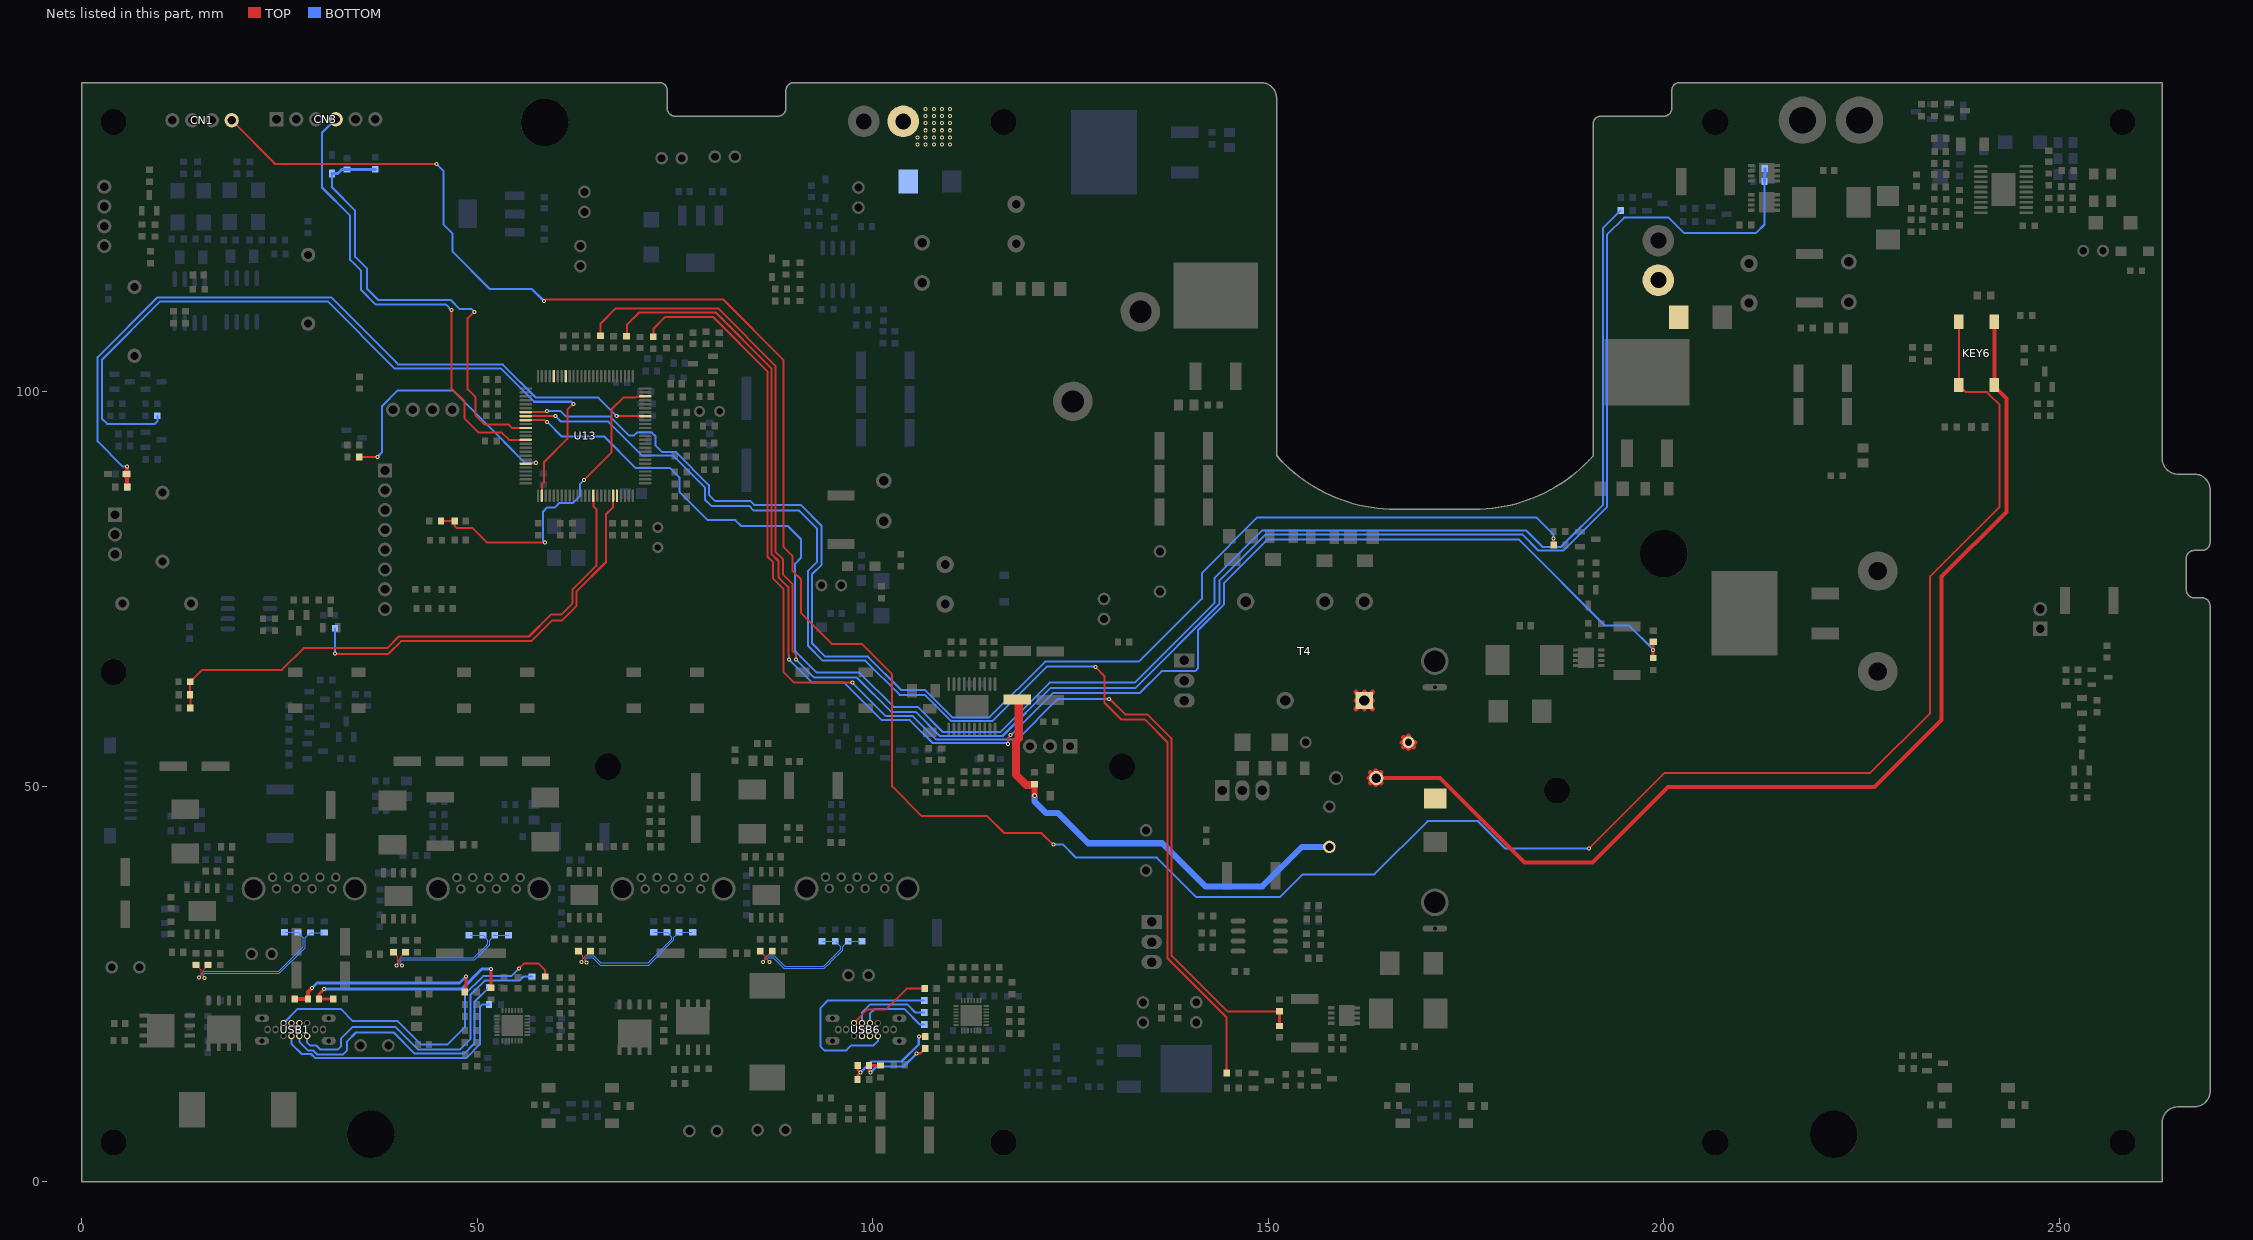
[diagram p0: the nets of this part, all layers, seen from the top]
# Altium PCB MISC84402.PcbDoc (part 4 of 12)
Units mm, origin at the board's own origin, x right, y up, seen from the top; angles counter-clockwise.
Board outline 269.06 x 139 mm, 4 copper layers (TOP, GND02, PWR03, BOTTOM), stack 0.732 mm thick; 694 components, 428 nets, 1859 pads, 1384 vias.

## Via types
v1: diameter 0.508, hole 0.254, TOP to BOTTOM, tented both sides, 1015 vias
v2: diameter 0.508, hole 0.254, TOP to BOTTOM, 243 vias
v3: diameter 0.508, hole 0.305, TOP to BOTTOM, 60 vias
v4: diameter 0.61, hole 0.305, TOP to BOTTOM, 55 vias
v5: diameter 0.61, hole 0.305, TOP to BOTTOM, tented both sides, 8 vias
v6: diameter 0.762, hole 0.381, TOP to BOTTOM, 2 vias
v7: diameter 0.762, hole 0.381, TOP to BOTTOM, tented both sides, 1 vias

## Nets (pads, with @x,y where several pads share a name; then routed paths per layer and width w, separated by ;. In a path a pad name is that pad's centre, name@x,y a point inside that pad or via, vN(x,y) a via of type N, cw(c..) or ccw(c..) an arc to the next point about the centre after c; other vN are vias at no path point) (continued)
BAT1+: C98.2 C125.1 F6.2 KEY6.3 KEY6.4 R13.2 R16.2 R20.1 T4.1 | length 218.9
  TOP w0.508: C98.2@163.906,51.105 171.679,51.105 182.397,40.386 190.983,40.386 200.508,49.911 226.644,49.911 235.128,58.395 235.128,76.556 243.307,84.734 243.307,99.06 241.798,100.569 KEY6.3@241.798,100.75 KEY6.4@241.798,108.75
  TOP w0.635: T4.1@161.074,59.82 T4.1@162.125,60.871 ; T4.1@161.074,60.871 T4.1@162.125,60.871 ; T4.1@161.074,61.922 T4.1@162.125,60.871 ; T4.1@162.125,59.82 T4.1@162.125,60.871 ; T4.1@162.125,61.922 T4.1@162.125,60.871 ; 162.725,51.095 C98.2@163.577,51.095 ; 162.924,50.442 C98.2@163.577,51.095 ; 162.924,51.748 C98.2@163.577,51.095 ; T4.1@163.176,59.82 T4.1@162.125,60.871 ; T4.1@163.176,60.871 T4.1@162.125,60.871 ; T4.1@163.176,61.922 T4.1@162.125,60.871 ; C98.2@163.577,50.243 C98.2@163.577,51.095 ; C98.2@163.577,51.946 C98.2@163.577,51.095 ; C98.2@164.229,50.442 C98.2@163.577,51.095 ; 164.229,51.748 C98.2@163.577,51.095 ; C98.2@164.428,51.095 C98.2@163.577,51.095 ; 166.899,55.591 R16.2@167.712,55.591 ; 167.086,54.965 R16.2@167.712,55.591 ; 167.086,56.217 R16.2@167.712,55.591 ; 167.712,54.777 R16.2@167.712,55.591 ; 167.712,56.404 R16.2@167.712,55.591 ; 168.338,54.965 R16.2@167.712,55.591 ; 168.525,55.591 R16.2@167.712,55.591
  TOP w0.762: v4(120.447,48.844) R20.1@120.447,50.14
  TOP w1.016: R13.2@118.238,60.983 118.44,60.78 118.44,56.058 118.11,55.728 118.11,51.486 119.431,50.165 R20.1@120.269,50.165
  BOTTOM w0.762: v4@120.447,48.793 120.447,48.082 121.895,46.634 123.419,46.634 127.229,42.824 136.576,42.824 142.037,37.363 149.25,37.363 154.254,42.367 C125.1@157.709,42.367
BAT-V: C59.2 R207.1 U13.23 | length 41.6
  TOP w0.254: R207.1@45.398,83.566 C59.2@47.114,83.566 47.114,82.934 47.371,82.677 49.403,82.677 51.206,80.874 57.734,80.874 v1(58.522,80.874) ; v1(63.5,88.773) 66.929,92.202 66.929,97.663 68.478,99.212 70.079,99.212 70.192,99.326 U13.23@71.203,99.326
  BOTTOM w0.254: v1(58.522,80.874) 58.293,81.102 58.293,84.734 58.852,85.293 59.817,85.293 60.376,85.852 62.103,85.852 62.992,86.741 62.992,88.265 v1(63.5,88.773)
BATA+: F1.1 J13.1
  other v1: 105.664,131.191 106.68,131.191 107.696,131.191 108.712,131.191 109.728,131.191 105.664,132.08 106.68,132.08 107.696,132.08 108.712,132.08 109.728,132.08 106.68,132.969 107.696,132.969 108.712,132.969 109.728,132.969 106.68,133.858 107.696,133.858 108.712,133.858 109.728,133.858 106.68,134.747 107.696,134.747 108.712,134.747 109.728,134.747 106.68,135.636 107.696,135.636 108.712,135.636 109.728,135.636
BATB+: F5.1 J1.1
BMS_EN: CN1.4 KEY6.1 KEY6.2 | length 356.2
  TOP w0.254: CN1.4@18.93,134.239 24.467,128.702 v2@44.755,128.702 ; v2@44.793,128.74 v2(44.831,128.702) ; v1@58.496,111.455 58.623,111.582 81.051,111.582 88.722,103.911 88.722,80.264 89.865,79.121 89.865,77.241 90.932,76.175 90.932,71.907 94.793,68.047 98.603,68.047 102.438,64.211 102.438,50.013 106.197,46.253 114.452,46.253 116.586,44.12 121.285,44.12 v1@122.784,42.621 ; v1@190.627,42.24 200.101,51.714 226.085,51.714 233.655,59.284 233.655,76.556 242.443,85.344 242.443,98.247 241.094,99.596 241.092,99.596 240.944,99.745 240.944,99.747 240.817,99.873 238.15,99.873 KEY6.1@237.465,100.559 ; KEY6.1@237.298,100.559 KEY6.1@237.298,100.75 KEY6.2@237.298,108.75
  BOTTOM w0.254: v2@44.907,128.626 45.687,127.846 45.687,126.289 ; 45.687,126.51 45.687,126.289 ; v1(58.42,111.379) 56.896,112.903 51.562,112.903 46.863,117.602 46.863,119.888 45.687,121.064 45.687,126.289 ; v1@122.809,42.697 v1(122.86,42.647) v1@122.872,42.634 ; v1@122.911,42.672 124.003,42.672 125.679,40.996 135.89,40.996 140.868,36.017 151.46,36.017 154.33,38.887 163.398,38.887 170.129,45.618 176.505,45.618 179.984,42.139 189.052,42.139 ; 189.509,42.139 189.052,42.139 ; v1@190.5,42.139 189.052,42.139
  other v1: 190.551,42.139
BUSY: C168.2 R321.1 R322.2 U13.90 | length 70.8
  TOP w0.254: R322.2@13.707,59.944 13.707,61.542 C168.2@13.654,61.595 13.654,63.193 R321.1@13.707,63.246 15.196,64.735 25.288,64.735 28.042,67.488 38.608,67.488 40.081,68.961 56.526,68.961 59.294,71.73 60.604,71.73 62.001,73.127 62.001,73.304 62.002,74.851 65.05,77.899 65.05,85.055 64.653,85.452 U13.90@64.653,86.776
CAR-EN: R191.1 U13.59 | length 216.5
  TOP w0.254: U13.59@56.103,96.326 56.957,96.326 56.965,96.318 58.486,96.318 58.7,96.104 v1(58.827,96.104)
  BOTTOM w0.254: v1(58.827,96.104) 60.68,94.251 66.023,94.251 69.977,90.297 74.29,90.297 75.565,89.022 75.565,87.198 79.096,83.668 82.601,83.668 83.337,82.931 89.23,82.931 90.907,81.255 90.907,78.918 90.17,78.181 90.17,67.132 90.246,67.056 ; 90.252,67.062 92.925,64.389 98.298,64.389 102.616,60.071 105.664,60.071 108.864,56.871 116.103,56.871 122.352,63.119 133.121,63.119 143.18,73.177 143.18,76.327 149.225,82.372 182.575,82.372 184.658,80.289 186.995,80.289 192.278,85.573 192.278,120.574 R191.1@194.488,122.784
CAR-I: C51.2 R67.2 R356.2 | length 250.9
  TOP w0.254: R356.2@65.557,107.213 65.557,108.509 67.488,110.439 80.442,110.439 87.681,103.2 87.681,79.68 88.646,78.715 88.646,76.785 89.815,75.616 89.815,67.157 90.297,66.675 v1(90.297,66.04)
  BOTTOM w0.254: v1(90.297,66.04) 92.565,63.772 97.987,63.772 102.323,59.436 105.41,59.436 108.458,56.388 116.383,56.388 122.428,62.433 133.172,62.433 143.815,73.076 143.815,76.022 149.631,81.839 152.578,81.839 152.756,81.839 182.143,81.839 184.15,79.832 187.3,79.832 192.786,85.319 192.786,119.736 194.97,121.92 200.609,121.92 202.54,119.99 211.658,119.99 212.725,121.056 212.725,121.412 C51.2@212.725,126.502
  BOTTOM w0.381: C51.2@212.725,126.502 212.725,127.329 212.778,127.382 R67.2@212.779,128.153
CC1-1: R164.1 USB6.A5 | length 27
  BOTTOM w0.254: USB6.A5@100.621,18.444 100.621,17.817 100.076,17.272 97.282,17.272 96.647,16.637 93.853,16.637 93.345,17.145 93.345,21.971 94.326,22.952 R164.1@106.472,22.952
CC1-2: R205.1 USB1.A5 | length 39.6
  BOTTOM w0.254: USB1.A5@28.48,18.444 28.48,17.621 28.829,17.272 29.591,17.272 30.099,16.764 32.385,16.764 32.766,17.145 32.766,18.161 34.188,19.583 39.65,19.583 42.47,16.764 47.803,16.764 49.098,18.059 49.098,23.637 50.917,25.456 55.301,25.456 55.827,25.982 R205.1@56.922,25.982
CC2-1: R160.1 USB6.B5 | length 10.5
  TOP w0.254: USB6.B5@97.815,20.345 99.289,21.819 101.676,21.819 104.333,24.476 R160.1@106.576,24.476
CC2-2: R203.1 USB1.B5 | length 43.5
  TOP w0.254: v1@55.27,27 55.905,27.635 57.699,27.635 58.573,26.762 R203.1@58.573,25.982
  BOTTOM w0.254: USB1.B5@25.48,20.094 27.23,21.844 32.766,21.844 34.265,20.345 39.904,20.345 42.851,17.399 46.228,17.399 48.412,19.583 48.412,23.713 50.734,26.035 54.29,26.035 v1(55.271,27.016)
CPC-1: R166.1 USB6.A6 USB6.B6 | length 12.1
  TOP w0.254: USB6.B6@98.621,20.094 98.621,19.444 USB6.A6@99.621,18.444
  BOTTOM w0.254: USB6.B6@98.621,20.094 98.621,21.405 99.67,22.454 104.343,22.454 105.369,21.428 R166.1@106.472,21.428
CPC-2: R204.1 USB1.A6 USB1.B6 | length 36.9
  BOTTOM w0.254: USB1.B6@26.48,20.094 27.48,19.094 USB1.A6@27.48,18.444 27.48,17.732 28.575,16.637 29.21,16.637 29.718,16.129 33.02,16.129 33.528,16.637 33.528,17.78 34.646,18.898 39.422,18.898 42.089,16.231 48.336,16.231 49.632,17.526 49.632,22.765 R204.1@51.47,24.603
CSNC1: C80.1 R116.1 R173.1 | length 10.6
  TOP w0.305: v1(105.537,16.256) 105.997,16.256 R173.1@106.596,16.856
  TOP w0.381: v1(99.695,13.843) 99.506,14.032 C80.1@99.506,14.732 R116.1@100.956,14.732
  BOTTOM w0.305: v1(99.695,13.843) 100.457,14.605 103.886,14.605 v1(105.537,16.256)
CSNC2: C91.1 R114.1 R213.1 | length 25
  TOP w0.381: R213.1@48.542,24.285 v1@48.542,25.908
  TOP w0.508: R114.1@26.924,23.114 C91.1@28.572,23.114 28.572,24 v1(29.083,24.511)
  BOTTOM w0.381: v1(29.083,24.511) 29.718,25.146 47.731,25.146 v1(48.567,25.982)
CSPC1: C80.2 R115.1 R170.1 | length 12.7
  TOP w0.305: R115.1@98.053,12.954 98.053,13.471 v1(98.425,13.843)
  TOP w0.381: C80.2@98.106,14.732 98.106,14.162 v1(98.425,13.843) ; v1(105.812,18.38) R170.1@106.596,18.38
  BOTTOM w0.305: v1(98.425,13.843) 99.811,15.229 103.621,15.229 105.812,17.42 v1(105.812,18.38)
  BOTTOM w0.381: v1(105.812,18.38) v1@105.817,18.375
CSPC2: C91.2 R113.1 R211.1 | length 28
  TOP w0.381: v1(30.607,24.384) 29.972,23.749 C91.2@29.972,23.114 R113.1@31.75,23.114 ; R211.1@51.715,24.638 v1(51.715,26.898)
  BOTTOM w0.381: v1(30.607,24.384) 40.386,24.384 ; 40.132,24.384 40.386,24.384 ; v1(51.715,26.898) 50.52,26.898 48.006,24.384 40.386,24.384
DC1-EN: R32.1 U13.58 | length 162
  TOP w0.254: U13.58@56.103,96.826 59.813,96.826 v1(59.843,96.856) ; v1(128.168,65.126) 128.168,65.075 129.286,63.957 129.286,60.579 131.369,58.496 134.367,58.496 137.236,55.627 137.236,28.321 144.704,20.853 R32.1@144.704,13.843
  BOTTOM w0.254: v1(59.843,96.856) 60.569,96.131 66.556,96.131 70.866,91.821 74.752,91.821 76.86,89.713 76.911,89.662 78.765,87.808 78.765,86.284 79.578,85.471 84.353,85.471 84.9,84.925 90.614,84.925 92.913,82.626 92.913,78.359 91.77,77.216 91.77,67.83 93.687,65.913 99.06,65.913 103.378,61.595 106.553,61.595 109.88,58.268 115.087,58.268 121.971,65.151 128.092,65.151 128.118,65.126 v1(128.168,65.126)
DC1-I: C53.2 R69.2 R354.2 | length 160.4
  TOP w0.254: R354.2@72.263,106.883 72.263,107.899 73.736,109.372 79.781,109.372 86.69,102.464 86.69,79.019 87.376,78.334 87.376,76.286 88.672,74.99 88.672,64.49 90.043,63.119 v1(97.409,63.119) ; v1(129.845,61.062) 129.845,60.96 v1@129.857,60.947 ; v1@129.972,61.062 131.902,59.131 134.661,59.131 137.77,56.023 137.77,28.6 144.806,21.564 R69.2@151.41,21.563
  TOP w0.381: C53.2@151.41,19.715 R69.2@151.41,21.563
  BOTTOM w0.254: v1(97.409,63.119) 101.635,58.893 105.064,58.893 108.026,55.931 118.237,55.931 123.393,61.087 v1@129.819,61.087
DC2-EN: R40.1 U13.57 | length 172.8
  TOP w0.254: U13.57@56.103,97.326 56.957,97.326 56.965,97.334 58.486,97.334 58.613,97.461 v1(58.827,97.461) ; v2(186.055,81.382) 186.06,81.377 R40.1@186.06,80.544
  BOTTOM w0.254: v1(58.827,97.461) 58.867,97.501 60.478,97.501 61.213,96.766 66.81,96.766 69.215,94.361 69.776,94.361 70.157,94.742 72.06,94.742 72.492,94.31 72.492,93.12 73.308,92.304 75.057,92.304 79.248,88.113 79.248,86.868 80.01,86.106 84.48,86.106 84.988,85.598 90.856,85.598 93.523,82.931 93.523,78.029 92.304,76.81 92.304,68.097 93.98,66.421 99.362,66.421 103.553,62.23 106.553,62.23 110.033,58.75 114.732,58.75 121.768,65.786 133.638,65.786 141.58,73.727 141.58,76.987 148.615,84.023 183.845,84.023 186.055,81.813 v2(186.055,81.382)
DC2-I: C56.2 R70.2 R355.2 | length 198
  TOP w0.254: R355.2@68.885,107.036 68.885,108.382 70.434,109.931 80.137,109.931 87.173,102.895 87.173,79.4 88.062,78.511 88.062,76.454 88.29,76.225 ; 88.295,76.23 89.307,75.218 89.307,66.649 89.408,66.548 v1(89.408,66.04) ; v2(117.069,55.372) 117.069,56.109 117.373,56.413 v2(117.373,56.49)
  TOP w0.381: R70.2@198.654,66.241 v1(198.654,67.275) C56.2@198.654,68.291
  BOTTOM w0.254: v1(89.408,66.04) 92.329,63.119 96.396,63.119 101.13,58.385 104.683,58.385 107.569,55.499 117.018,55.499 v2@117.069,55.448 ; v2(117.373,56.49) 117.45,56.49 122.758,61.798 133.706,61.798 136.5,64.592 140.767,64.592 141.097,64.922 141.097,69.367 141.097,69.52 141.097,69.723 144.374,73 144.374,75.692 149.936,81.255 181.635,81.255 192.557,70.333 195.631,70.333 v1@198.628,67.335 ; v1(198.654,67.275) v1@198.654,67.335
DM1: C183.2 R97.1 R243.1 | length 20.5
  TOP w0.127: R243.1@14.431,27.427 15.062,26.795 15.062,26.086 v2(14.808,25.832)
  BOTTOM w0.127: v2@14.884,25.883 15.062,26.06 15.062,26.289 15.392,26.619 24.863,26.619 27.991,29.747 27.991,30.124 ; C183.2@25.73,31.547 R97.1@27.331,31.547 27.991,30.887 27.991,30.124 ; 27.991,30.103 27.991,30.124
DM2: C185.2 R89.1 R120.1 | length 17.8
  TOP w0.127: R89.1@39.396,29.065 39.954,28.507 39.954,27.534 v2@39.802,27.381
  BOTTOM w0.127: 39.98,27.534 39.98,27.94 40.056,28.016 40.056,28.02 40.357,28.321 49.526,28.321 51.103,29.898 ; C185.2@49.124,31.166 R120.1@50.733,31.166 ; R120.1@50.698,31.2 R120.1@50.733,31.166 ; R120.1@50.775,31.166 R120.1@50.733,31.166 ; 51.232,30.026 51.103,29.898 ; R120.1@50.733,31.166 51.308,30.59 51.308,30.103 51.103,29.898
  other v2: 39.776,27.356
DM3: C180.2 R84.1 R111.1 | length 17.7
  TOP w0.127: R111.1@62.764,29.192 63.348,28.608 v2@63.348,27.965
  BOTTOM w0.127: v2@63.17,27.813 63.348,27.991 63.348,28.245 63.373,28.27 63.373,28.274 63.7,28.6 64.697,28.6 65.612,27.686 71.574,27.686 74.6,30.712 74.6,30.963 73.981,31.581 R84.1@73.965,31.581 ; C180.2@72.298,31.566 R84.1@73.844,31.566
  other v2: 63.17,27.788
DM4: C187.2 R137.1 R247.1 | length 16
  TOP w0.127: R247.1@85.751,29.192 86.411,28.532 86.411,28.143 v2(86.106,27.838)
  BOTTOM w0.127: v2@86.208,27.915 86.411,28.118 86.411,28.375 86.661,28.626 87.507,28.626 88.853,27.28 93.773,27.28 95.91,29.417 95.91,29.752 R137.1@95.25,30.413 ; C187.2@93.583,30.423 R137.1@95.002,30.423
DMC-1: R167.1 USB6.A7 USB6.B7 | length 11.1
  BOTTOM w0.254: USB6.A7@98.621,18.444 98.621,19.094 USB6.B7@99.621,20.094 99.621,21.262 100.203,21.844 104.013,21.844 105.953,19.904 R167.1@106.472,19.904
DMC-2: R208.1 USB1.A7 USB1.B7 | length 34.6
  TOP w0.254: USB1.A7@26.48,18.444 26.48,19.094 USB1.B7@27.48,20.094
  BOTTOM w0.254: USB1.A7@26.48,18.444 26.48,17.488 27.788,16.18 28.956,16.18 29.489,15.646 48.565,15.646 50.317,17.399 50.317,21.717 ; 50.317,21.936 50.317,21.717 ; R208.1@51.47,22.444 50.638,22.444 50.317,22.123 50.317,21.717
DP1: C182.2 R92.1 R242.1 | length 20.5
  TOP w0.127: v2(15.519,25.806) 15.316,26.01 15.316,26.788 R242.1@15.955,27.427
  BOTTOM w0.127: v2@15.418,25.908 15.316,26.01 15.316,26.184 15.498,26.365 24.968,26.365 28.245,29.642 28.245,30.15 ; 28.245,29.997 28.245,30.15 ; C182.2@30.462,31.539 R92.1@28.905,31.539 28.245,30.879 28.245,30.15
DP2: C184.2 R81.1 R102.1 | length 17.7
  TOP w0.127: v2@40.259,27.534 40.259,28.404 R81.1@40.92,29.065
  BOTTOM w0.127: v2@40.361,27.407 40.234,27.534 40.234,27.835 40.31,27.911 40.31,27.915 40.462,28.067 49.632,28.067 51.321,29.756 ; 51.486,29.921 51.321,29.756 ; R102.1@51.918,30.937 51.562,30.582 51.562,29.997 51.321,29.756 ; R102.1@52.025,31.211 C184.2@53.933,31.211
  other v2: 40.437,27.356
DP3: C181.2 R90.1 R238.1 | length 17.5
  TOP w0.127: v2@63.627,27.94 63.627,28.531 R238.1@64.288,29.192
  BOTTOM w0.127: v2(63.805,27.762) 63.627,27.94 63.627,28.169 63.805,28.346 64.592,28.346 65.507,27.432 71.679,27.432 74.854,30.607 74.854,30.963 R90.1@75.235,31.344 ; R90.1@75.489,31.59 C181.2@77.097,31.59
DP4: C186.2 R123.1 R245.1 | length 15.7
  TOP w0.127: v2(86.944,27.838) 86.665,28.118 86.665,28.582 R245.1@87.275,29.192
  BOTTOM w0.127: v2(86.944,27.838) 86.665,28.118 86.665,28.27 86.766,28.372 87.401,28.372 88.748,27.026 93.878,27.026 94.59,27.737 94.729,27.877 96.164,29.312 96.164,29.769 R123.1@96.52,30.124 ; R123.1@96.891,30.421 C186.2@98.357,30.421
EN9V-INT: C2.2 D11.1 R270.2 U13.61 | length 58.2
  TOP w0.254: v1@49.53,109.982 48.768,109.22 48.768,100.203 49.784,99.187 49.784,96.901 50.927,95.758 53.975,95.758 54.407,95.326 U13.61@56.103,95.326
  BOTTOM w0.254: D11.1@31.623,127.508 31.623,125.73 34.544,122.809 34.544,116.967 36.068,115.443 36.068,112.903 37.465,111.506 46.609,111.506 47.752,110.363 48.641,110.363 ; 49.149,110.363 48.641,110.363 ; v1(49.657,109.982) 49.276,110.363 48.641,110.363
  BOTTOM w0.381: D11.1@31.623,127.508 32.333,127.508 32.841,128.016 C2.2@33.528,128.016 ; C2.2@33.546,128.034 35.306,128.034 R270.2@37.084,128.034
EN_485_INV: R176.1 U13.70 | length 34.4
  TOP w0.254: R176.1@35.078,91.659 v1(37.364,91.659) ; U13.70@56.103,90.826 57.296,90.826 v1(57.403,90.932)
  BOTTOM w0.254: v1(37.364,91.659) 37.94,92.235 37.94,98.077 39.939,100.076 46.88,100.076 53.385,93.571 53.385,93.554 56.007,90.932 v1(57.403,90.932)
EN_BMS_IN: R184.1 U13.77 | length 96.8
  TOP w0.254: U13.77@58.153,86.776 58.153,88.191 58.446,88.484 58.446,91.024 61.367,93.945 61.367,97.628 v1(62.129,98.39)
  BOTTOM w0.254: R184.1@9.542,96.866 9.542,96.156 9.236,95.85 3.2,95.85 2.54,96.51 2.54,103.952 9.925,111.337 31.055,111.337 39.558,102.835 52.994,102.835 57.185,98.644 61.875,98.644 v1(62.129,98.39)
EN_BMS_OUT: U13.46
EN_INV: CN3.4 U13.64 | length 60.1
  TOP w0.254: v1(46.711,110.236) 46.711,100.355 48.387,98.679 48.387,96.52 50.165,94.742 53.086,94.742 54.002,93.826 U13.64@56.103,93.826
  BOTTOM w0.254: CN3.4@32.091,134.366 30.353,132.628 30.353,125.73 33.909,122.174 33.909,116.586 35.306,115.189 35.306,112.776 37.169,110.913 46.034,110.913 v1(46.711,110.236)
FAN1: C93.2 D57.1 R276.2 R298.2 U13.18 | length 99.6
  TOP w0.254: R298.2@5.643,87.928 R298.2@5.723,87.849 ; v1@5.643,90.365 5.643,90.416 v1(5.679,90.451) ; v1@67.616,96.826 U13.18@71.203,96.826
  TOP w0.508: R298.2@5.723,87.849 v1@5.723,90.365
  BOTTOM w0.254: v1@5.679,90.399 v1(5.679,90.451) 5.171,90.451 1.981,93.64 1.981,104.282 9.551,111.852 31.522,111.852 39.734,103.64 ; 39.726,103.632 40.015,103.343 53.213,103.343 57.404,99.152 65.289,99.152 v1(67.615,96.826)
  BOTTOM w0.508: v1@5.69,90.399 5.69,87.891 R276.2@5.732,87.849
FAN1-EN: R186.1 U13.95 | length 52.1
  TOP w0.254: v2@32.029,66.777 38.76,66.777 40.361,68.377 56.83,68.377 59.447,70.993 60.706,70.993 62.509,72.796 62.509,73.101 62.51,74.641 66.256,78.387 66.256,84.417 67.153,85.314 U13.95@67.153,86.776
  BOTTOM w0.254: v2(31.995,66.785) R186.1@31.995,70.002
FAN2: U13.43
FAN2-EN: U13.96